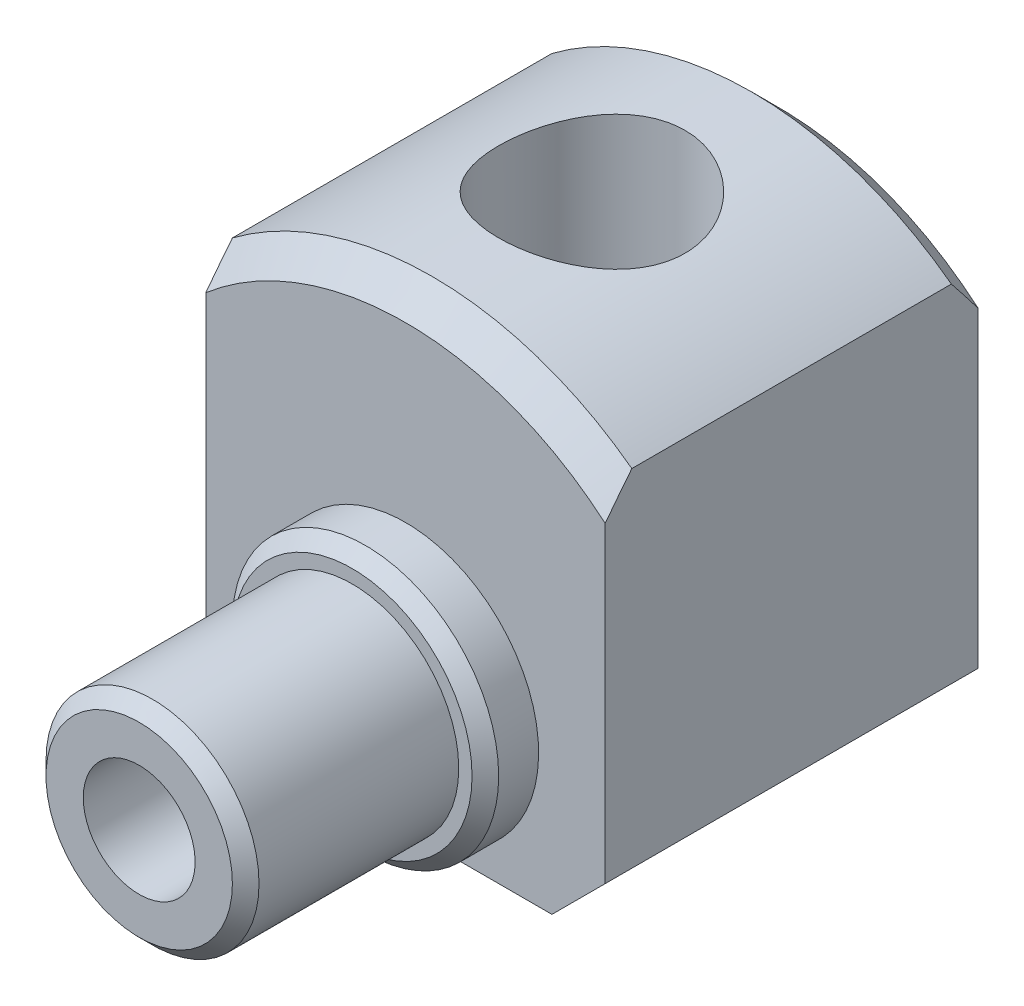
from build123d import *

# Parameters (mm, degrees)
SKETCH1_R           = 12.5
BOSS_EXTRUDE1_DEPTH = 12
SKETCH2_OUTSIDE_W   = 35.546
SKETCH2_OUTSIDE_H   = 35.546
SKETCH2_OUTSIDE_R   = 4
CUT_EXTRUDE1_DEPTH  = 10
SKETCH9_OUTSIDE_W   = 35.546
SKETCH9_OUTSIDE_H   = 35.546
SKETCH9_OUTSIDE_W_2 = 15
SKETCH9_OUTSIDE_H_2 = 20
CUT_EXTRUDE2_DEPTH  = 30.807717122
M5_TAPPED_HOLE1_D   = 4.2
BOSS_EXTRUDE2_START = 2
SKETCH8_R           = 5
SKETCH8_R_2         = 4
BOSS_EXTRUDE2_DEPTH = 2
SKETCH6_W           = 3.5
SKETCH6_H           = 12.5
CHAMFER1_SIZE       = 0.5
CHAMFER2_SIZE       = 2
CHAMFER3_SIZE       = 1


with BuildPart() as part:
    # Sketch1 → Boss-Extrude1 (new, symmetric)
    with BuildSketch(Plane.XY):
        Circle(SKETCH1_R)
    extrude(amount=BOSS_EXTRUDE1_DEPTH, both=True)

    # Sketch2 outside → Cut-Extrude1 (cut)
    with BuildSketch(Plane.XY.offset(12)):
        Rectangle(SKETCH2_OUTSIDE_W, SKETCH2_OUTSIDE_H)
        Circle(SKETCH2_OUTSIDE_R, mode=Mode.SUBTRACT)
    extrude(amount=-CUT_EXTRUDE1_DEPTH, mode=Mode.SUBTRACT)

    # Sketch9 outside → Cut-Extrude2 (cut, through all)
    with BuildSketch(Plane(origin=(0, 0, -12), x_dir=(-1, 0, 0), z_dir=(0, 0, -1))):
        Rectangle(SKETCH9_OUTSIDE_W, SKETCH9_OUTSIDE_H)
        with Locations((0, 5)):
            Rectangle(SKETCH9_OUTSIDE_W_2, SKETCH9_OUTSIDE_H_2, mode=Mode.SUBTRACT)
    extrude(amount=-CUT_EXTRUDE2_DEPTH, mode=Mode.SUBTRACT)

    # M5 Tapped Hole1 (through all)
    with Locations(Plane(origin=(0, 0, -12), x_dir=(-1, 0, 0), z_dir=(0, 0, -1))):
        with Locations((0, 0)):
            Hole(M5_TAPPED_HOLE1_D / 2)

    # Sketch8 → Boss-Extrude2 (add)
    with BuildSketch(Plane.XY.offset(2).offset(BOSS_EXTRUDE2_START)):
        with Locations(Location((0, 0, 0), (0, 0, 270))):
            Circle(SKETCH8_R)
        Circle(SKETCH8_R_2, mode=Mode.SUBTRACT)
    extrude(amount=-BOSS_EXTRUDE2_DEPTH)

    # Sketch6 → M8x1.0 Tapped Hole1 (revolve, cut)
    with BuildSketch(Plane(origin=(0, 0, -5), x_dir=(0, 0, -1), z_dir=(1, 0, 0))):
        with Locations((1.75, 6.25)):
            Rectangle(SKETCH6_W, SKETCH6_H)
    revolve(axis=Axis((0, -6.35, -5), (0, 1, 0)), mode=Mode.SUBTRACT)

    # Chamfer1
    chamfer1_edges = [part.edges().sort_by_distance(p)[0] for p in [
        (-4, 0, 12),
        (0, 5, 4),
    ]]
    chamfer(chamfer1_edges, length=CHAMFER1_SIZE)

    # Chamfer2
    chamfer2_edges = [part.edges().sort_by_distance(p)[0] for p in [
        (-7.5, -5, -5),
        (7.5, -5, -5),
    ]]
    chamfer(chamfer2_edges, length=CHAMFER2_SIZE)

    # Chamfer3
    chamfer3_edges = [part.edges().sort_by_distance(p)[0] for p in [
        (0, 12.5, -12),
        (0, 12.5, 2),
    ]]
    chamfer(chamfer3_edges, length=CHAMFER3_SIZE)


solid = part.part
